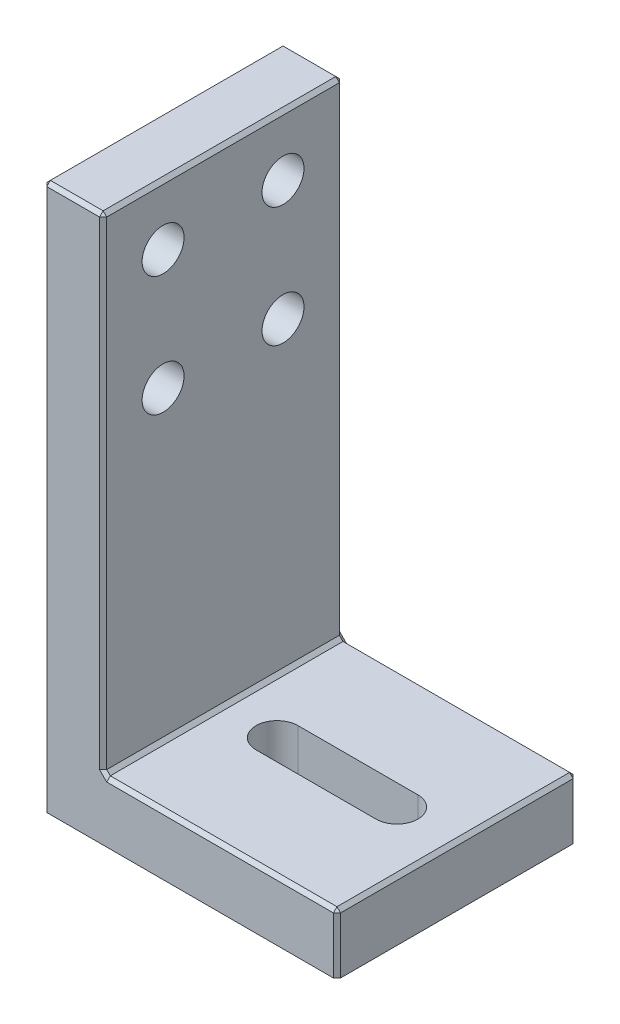
SolidWorks part; units mm, degrees
ref_plane "Front Plane" through (0, 0, 0) normal (0, 0, 1) x (1, 0, 0)
ref_plane "Top Plane" through (0, 0, 0) normal (0, 1, 0) x (1, 0, 0)
ref_plane "Right Plane" through (0, 0, 0) normal (1, 0, 0) x (0, 0, -1)
sketch "Sketch1" plane through (0, 0, 0) normal (0, 0, 1) x (1, 0, 0)
  line L0 (0, 45.5) -> (0, 0)
  line L1 (0, 0) -> (24.5, 0)
  dimension "D1" = 24.5
  dimension "D2" = 45.5
extrude "Extrude-Thin1" add sketch "Sketch1" along normal blind 20 thin thin type one direction reverse wall 5
chamfer "Chamfer1" distance 0.3 angle 45 15 edges at (24.5, 5, 10) (24.5, 2.5, 0) (14.75, 5, 0) (5, 5, 10) (5, 25.25, 0) (0, 22.75, 20) (0, 0, 10) (0, 22.75, 0) (5, 45.5, 10) (2.5, 45.5, 0) (0, 45.5, 10) (2.5, 45.5, 20) (5, 25.25, 20) (14.75, 5, 20) (24.5, 2.5, 20)
sketch "Sketch2" plane through (0, 5, 0) normal (0, 1, 0) x (1, 0, 0)
  line L0 (24.2, -10) -> (-5.965, -10) construction
  line L1 (24.2, -19.7) -> (24.2, -0.3) construction
  line L2 (9.5, -10) -> (19.5, -10) construction
  line L3 (9.5, -8.25) -> (19.5, -8.25)
  line L4 (9.5, -11.75) -> (19.5, -11.75)
  line L5 (24.5, -0.3) -> (24.5, -19.7) construction
  arc A0 (9.5, -8.25) -> (9.5, -11.75) centre (9.5, -10) ccw
  arc A1 (19.5, -11.75) -> (19.5, -8.25) centre (19.5, -10) ccw
  point P6 (14.5, -10)
  dimension "D2" = 1.75
  dimension "D3" = 5
  dimension "D1" = 10
extrude "Cut-Extrude1" cut sketch "Sketch2" against normal up to next
sketch "Sketch3" plane through (5, 0, 0) normal (1, 0, 0) x (0, 0, -1)
  line L0 (-10, 62.1837) -> (-10, -20.3146) construction
  line L1 (-19.7, 45.5) -> (-0.3, 45.5) construction
  line L3 (-20, 5.3) -> (-20, 45.2) construction
  circle A0 centre (-15, 40.5) radius 1.75
  circle A1 centre (-15, 30.5) radius 1.75
  circle A2 centre (-5, 30.5) radius 1.75
  circle A3 centre (-5, 40.5) radius 1.75
  dimension "D1" = 3.5
  dimension "D2" = 5
  dimension "D3" = 5
  dimension "D4" = 10
extrude "Cut-Extrude2" cut sketch "Sketch3" against normal up to next
